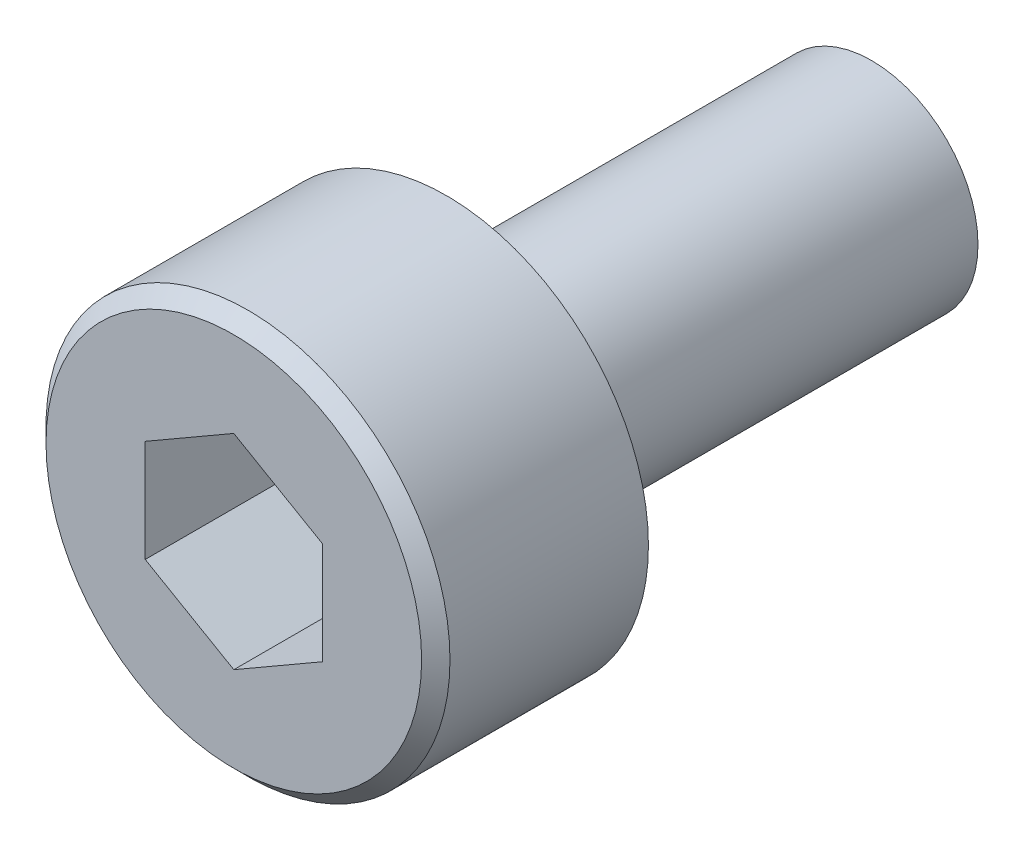
SolidWorks part; units mm, degrees
ref_plane "前视基准面" through (0, 0, 0) normal (0, 0, 1) x (1, 0, 0)
ref_plane "上视基准面" through (0, 0, 0) normal (0, 1, 0) x (1, 0, 0)
ref_plane "右视基准面" through (0, 0, 0) normal (1, 0, 0) x (0, 0, -1)
sketch "草图1" plane through (0, 0, 0) normal (0, 0, 1) x (1, 0, 0)
  circle A0 centre (0, 0) radius 2.85
  dimension "D1" = 5.7
extrude "凸台-拉伸1" add sketch "草图1" along normal blind 3
sketch "草图2" plane through (0, 0, 3) normal (0, 0, 1) x (1, 0, 0)
  line L1 (0, 1.4434) -> (-1.25, 0.7217)
  line L2 (-1.25, 0.7217) -> (-1.25, -0.7217)
  line L3 (-1.25, -0.7217) -> (0, -1.4434)
  line L4 (0, -1.4434) -> (1.25, -0.7217)
  line L5 (1.25, -0.7217) -> (1.25, 0.7217)
  line L6 (1.25, 0.7217) -> (0, 1.4434)
  circle A0 centre (0, 0) radius 1.25 construction
  dimension "D1" = 2.5
extrude "切除-拉伸1" cut sketch "草图2" against normal blind 4
chamfer "倒角1" distance 0.2 angle 45 1 edges at (2.85, 0, 3)
sketch "草图3" plane through (0, 0, 0) normal (0, 0, -1) x (-1, 0, 0)
  circle A0 centre (0, 0) radius 1.5
  dimension "D1" = 3
extrude "凸台-拉伸2" add sketch "草图3" along normal blind 6
cosmetic thread "装饰螺纹线1" parameters "D2"=2.459
